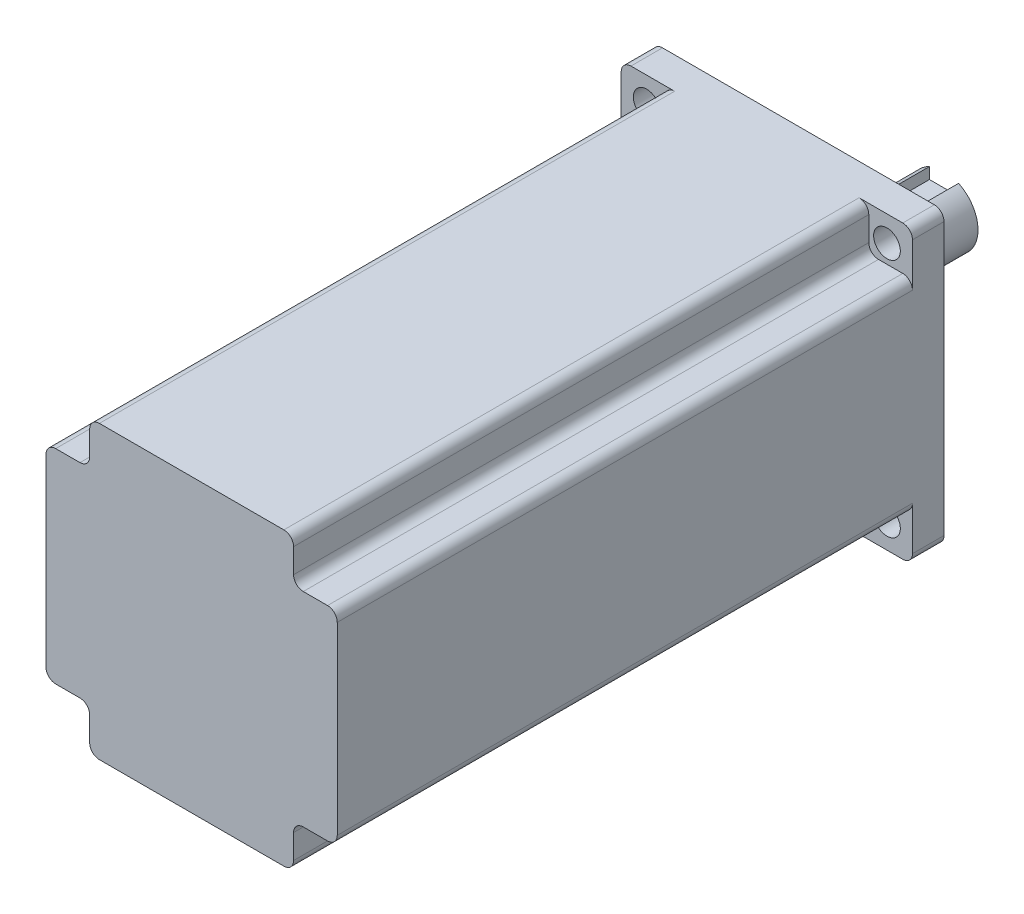
from build123d import *

# Parameters (mm, degrees)
SKETCH_1_W                  = 60
SKETCH_1_H                  = 60
EXTRUDE_1_DEPTH             = 125
SKETCH_2_R                  = 25
EXTRUDE_2_DEPTH             = 3
SKETCH_3_R                  = 7
EXTRUDE_3_DEPTH             = 27
CUT_EXTRUDE_1_DEPTH         = 3
HOLE_WIZARD_M5_1_D          = 4.2
HOLE_WIZARD_M5_1_DEPTH      = 6
HOLE_WIZARD_M5_1_TIP        = 1.2618073
HOLE_WIZARD_4_5_4_5_1_D     = 5.5
HOLE_WIZARD_4_5_4_5_1_DEPTH = 10
HOLE_WIZARD_4_5_4_5_1_TIP   = 1.652366702
SKETCH_10_W                 = 9
SKETCH_10_H                 = 9
CUT_EXTRUDE_2_DEPTH         = 118.5
MIRROR_2_COPY_1_SKETCH_W    = 9
MIRROR_2_COPY_1_SKETCH_H    = 9
MIRROR_2_COPY_1_DEPTH       = 118.5
FILLET_1_R                  = 2


with BuildPart() as part:
    # 草图1 → 凸台-拉伸1 (new body)
    with BuildSketch(Plane.XY):
        Rectangle(SKETCH_1_W, SKETCH_1_H)
    extrude(amount=EXTRUDE_1_DEPTH)

    # 草图2 → 凸台-拉伸2 (add)
    with BuildSketch(Plane(origin=(0, 0, 0), x_dir=(-1, 0, 0), z_dir=(0, 0, -1))):
        with Locations(Location((0, 0, 0), (0, 0, 180))):
            Circle(SKETCH_2_R)
    extrude(amount=EXTRUDE_2_DEPTH)

    # 草图3 → 凸台-拉伸3 (add)
    with BuildSketch(Plane(origin=(0, 0, -3), x_dir=(-1, 0, 0), z_dir=(0, 0, -1))):
        Circle(SKETCH_3_R)
    extrude(amount=EXTRUDE_3_DEPTH)

    # 草图4 → 切除-拉伸1 (cut)
    with BuildSketch(Plane(origin=(0, 7, 0), x_dir=(1, 0, 0), z_dir=(0, 1, 0))):
        with BuildLine():
            Line((3, 30), (3, 7.5))
            ThreePointArc((3, 7.5), (0, 4.5), (-3, 7.5))
            Line((-3, 7.5), (-3, 30))
            ThreePointArc((-3, 30), (0, 33), (3, 30))
        make_face()
    extrude(amount=-CUT_EXTRUDE_1_DEPTH, mode=Mode.SUBTRACT)

    # M5 螺纹孔1
    with Locations(Plane(origin=(0, 0, -30), x_dir=(-1, 0, 0), z_dir=(0, 0, -1))):
        with Locations((0, 0)):
            Hole(HOLE_WIZARD_M5_1_D / 2, depth=HOLE_WIZARD_M5_1_DEPTH)
            with Locations((0, 0, -(HOLE_WIZARD_M5_1_DEPTH + HOLE_WIZARD_M5_1_TIP / 2))):  # 118° drill point
                Cone(0, HOLE_WIZARD_M5_1_D / 2, HOLE_WIZARD_M5_1_TIP, mode=Mode.SUBTRACT)

    # Ø4.5 (4.5) 直径孔1
    with Locations(Plane(origin=(0, 0, 0), x_dir=(-1, 0, 0), z_dir=(0, 0, -1))):
        with Locations((-24.748737342, 24.748737342), (24.748737342, 24.748737342), (24.748737342, -24.748737342), (-24.748737342, -24.748737342)):
            Hole(HOLE_WIZARD_4_5_4_5_1_D / 2, depth=HOLE_WIZARD_4_5_4_5_1_DEPTH)
            with Locations((0, 0, -(HOLE_WIZARD_4_5_4_5_1_DEPTH + HOLE_WIZARD_4_5_4_5_1_TIP / 2))):  # 118° drill point
                Cone(0, HOLE_WIZARD_4_5_4_5_1_D / 2, HOLE_WIZARD_4_5_4_5_1_TIP, mode=Mode.SUBTRACT)

    # 草图10 → 切除-拉伸2 (cut)
    with BuildSketch(Plane.XY.offset(125)):
        with Locations((-25.5, 25.5)):
            Rectangle(SKETCH_10_W, SKETCH_10_H)
    cut_extrude_2 = extrude(amount=-CUT_EXTRUDE_2_DEPTH, mode=Mode.SUBTRACT)

    # 镜向1: 切除-拉伸2 across plane
    add(cut_extrude_2.mirror(Plane(origin=(0, 0, 0), x_dir=(0, 0, 1), z_dir=(1, 0, 0))), mode=Mode.SUBTRACT)

    # 镜向2: 切除-拉伸2 across plane
    add(cut_extrude_2.mirror(Plane.ZX), mode=Mode.SUBTRACT)

    # 镜向2 copy 1 sketch → 镜向2 copy 1 (cut)
    with BuildSketch(Plane(origin=(0, 0, 125), x_dir=(-1, 0, 0), z_dir=(0, 0, 1))):
        with Locations((-25.5, 25.5)):
            Rectangle(MIRROR_2_COPY_1_SKETCH_W, MIRROR_2_COPY_1_SKETCH_H)
    extrude(amount=-MIRROR_2_COPY_1_DEPTH, mode=Mode.SUBTRACT)

    # 圆角1
    fillet_1_edges = [part.edges().sort_by_distance(p)[0] for p in [
        (-30, -30, 3.25),
        (-30, -21, 65.75),
        (-21, -21, 65.75),
        (-21, -30, 65.75),
        (-30, 30, 3.25),
        (-30, 21, 65.75),
        (-21, 30, 65.75),
        (-21, 21, 65.75),
        (30, 30, 3.25),
        (30, 21, 65.75),
        (21, 21, 65.75),
        (21, 30, 65.75),
        (30, -30, 3.25),
        (30, -21, 65.75),
        (21, -30, 65.75),
        (21, -21, 65.75),
    ]]
    fillet(fillet_1_edges, radius=FILLET_1_R)


solid = part.part
